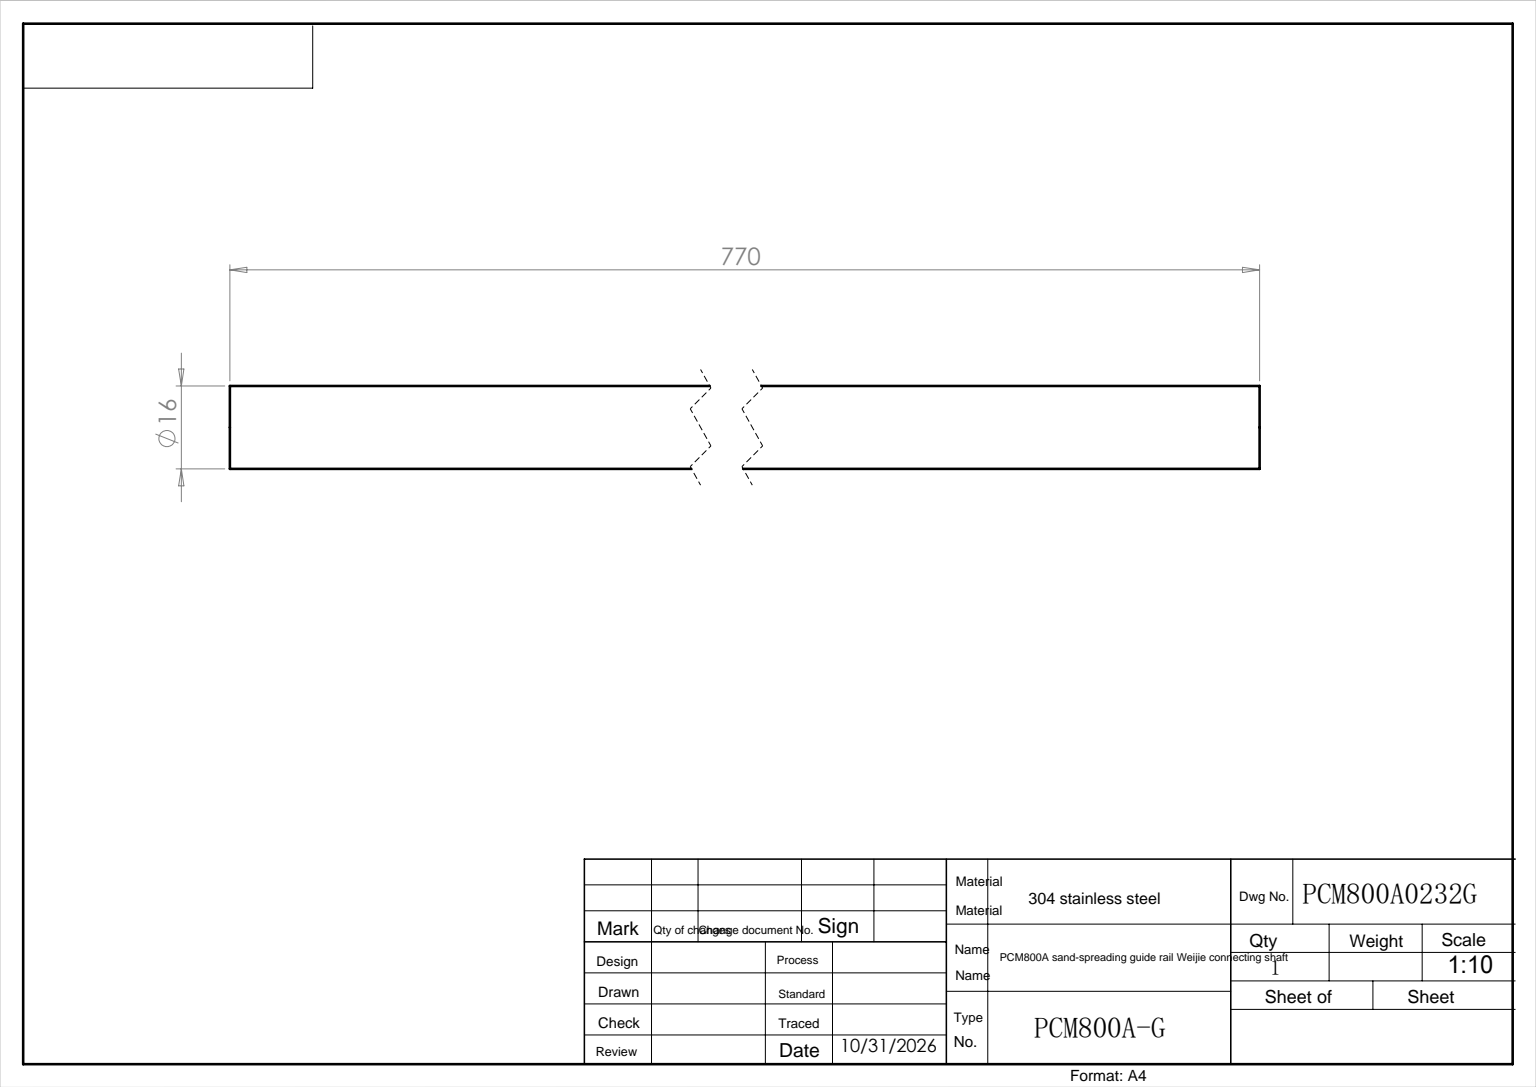
from build123d import *

# Parameters (mm, degrees)
SKETCH_1_R        = 8
EXTRUDE_207_DEPTH = 770


with BuildPart() as part:
    # 草图1 → Extrude 207 (new body)
    with BuildSketch(Plane.XY):
        Circle(SKETCH_1_R)
    extrude(amount=EXTRUDE_207_DEPTH)


solid = part.part
